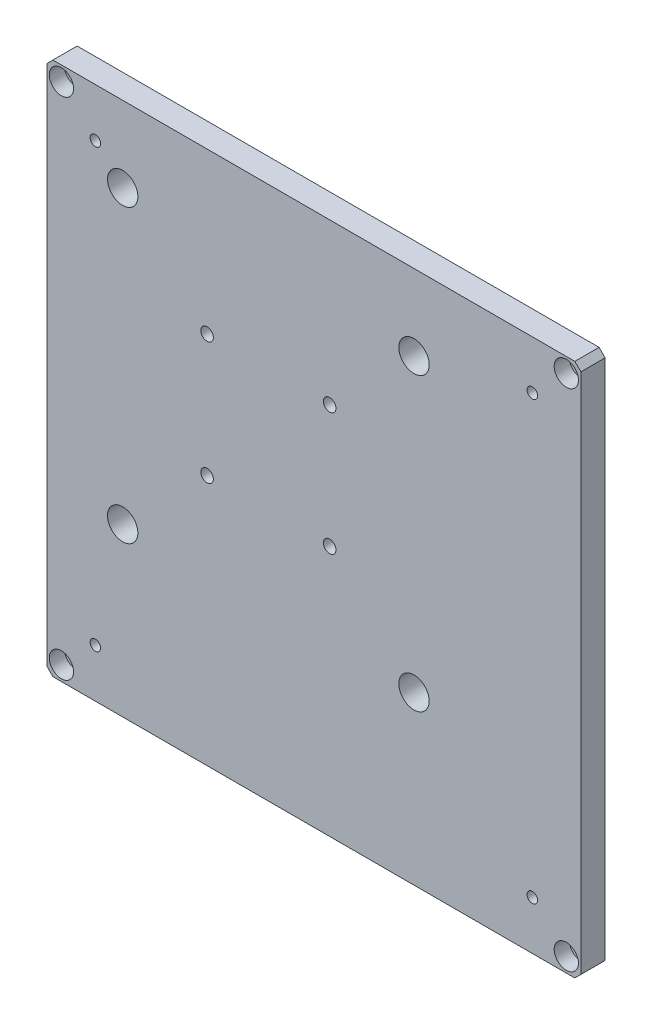
from build123d import *

# Parameters (mm, degrees)
SKETCH1_R           = 8.647
SKETCH1_R_2         = 13
SKETCH1_R_3         = 10.376
SKETCH1_R_4         = 25
BOSS_EXTRUDE1_DEPTH = 40
SKETCH2_R           = 20
CUT_EXTRUDE1_DEPTH  = 25


with BuildPart() as part:
    # Sketch1 → Boss-Extrude1 (new body)
    with BuildSketch(Plane.XY):
        Polygon((498.749353033, 365), (-361.250646967, 365), (-371.250646967, 355), (-371.250646967, -505), (-361.250646967, -515), (498.749353033, -515), (508.749353033, -505), (508.749353033, 355), align=None)
        with Locations((428.749353033, -435)):
            Circle(SKETCH1_R, mode=Mode.SUBTRACT)
        with Locations((-291.250646967, 285)):
            Circle(SKETCH1_R, mode=Mode.SUBTRACT)
        with Locations((428.749353033, 285)):
            Circle(SKETCH1_R, mode=Mode.SUBTRACT)
        with Locations((-291.250646967, -435)):
            Circle(SKETCH1_R, mode=Mode.SUBTRACT)
        with Locations((484.749353033, -491)):
            Circle(SKETCH1_R_2, mode=Mode.SUBTRACT)
        with Locations((-347.250646967, 341)):
            Circle(SKETCH1_R_2, mode=Mode.SUBTRACT)
        with Locations((484.749353033, 341)):
            Circle(SKETCH1_R_2, mode=Mode.SUBTRACT)
        with Locations((-347.250646967, -491)):
            Circle(SKETCH1_R_2, mode=Mode.SUBTRACT)
        with Locations((-107.250646967, -101)):
            Circle(SKETCH1_R_3, mode=Mode.SUBTRACT)
        with Locations((94.749353033, 101)):
            Circle(SKETCH1_R_3, mode=Mode.SUBTRACT)
        with Locations((-107.250646967, 101)):
            Circle(SKETCH1_R_3, mode=Mode.SUBTRACT)
        with Locations((94.749353033, -101)):
            Circle(SKETCH1_R_3, mode=Mode.SUBTRACT)
        with Locations((-246.250646967, -240)):
            Circle(SKETCH1_R_4, mode=Mode.SUBTRACT)
        with Locations((233.749353033, 240)):
            Circle(SKETCH1_R_4, mode=Mode.SUBTRACT)
        with Locations((-246.250646967, 240)):
            Circle(SKETCH1_R_4, mode=Mode.SUBTRACT)
        with Locations((233.749353033, -240)):
            Circle(SKETCH1_R_4, mode=Mode.SUBTRACT)
    extrude(amount=BOSS_EXTRUDE1_DEPTH)

    # Sketch2 → Cut-Extrude1 (cut)
    with BuildSketch(Plane.XY.offset(40)):
        with Locations((-347.250646967, 341)):
            Circle(SKETCH2_R)
        with Locations((484.749353033, 341)):
            Circle(SKETCH2_R)
        with Locations((484.749353033, -491)):
            Circle(SKETCH2_R)
        with Locations((-347.250646967, -491)):
            Circle(SKETCH2_R)
    extrude(amount=-CUT_EXTRUDE1_DEPTH, mode=Mode.SUBTRACT)


solid = part.part
